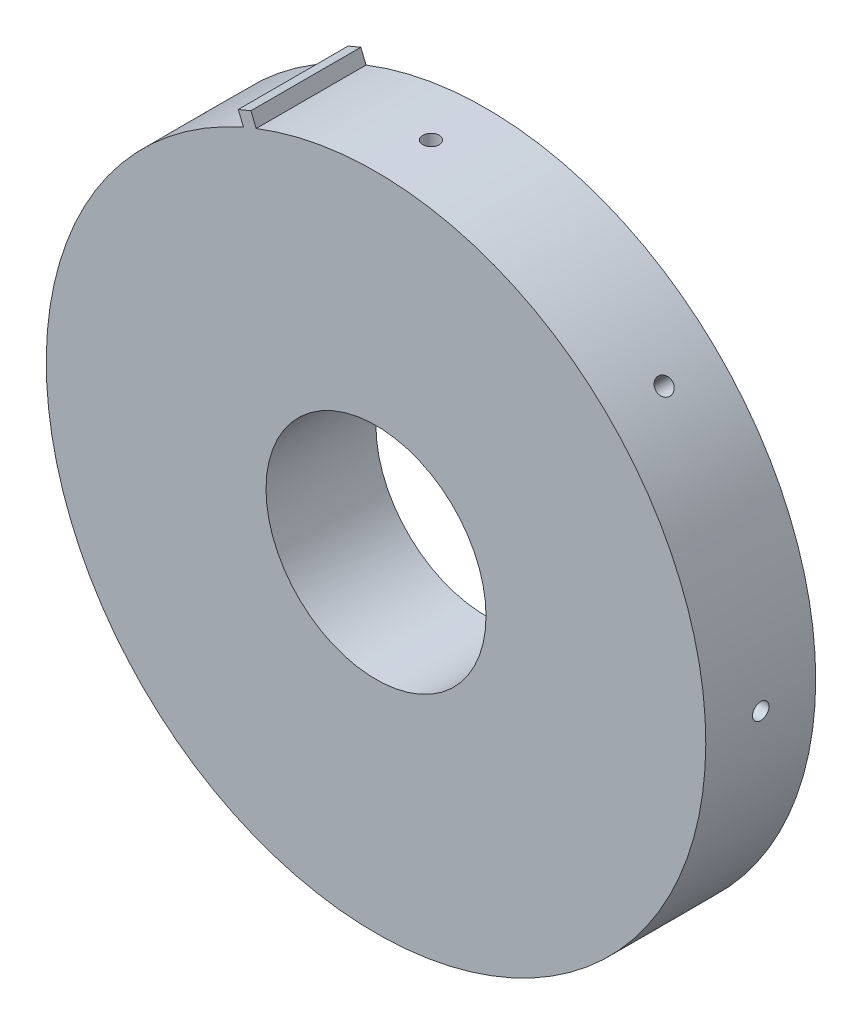
SolidWorks part; units mm, degrees
ref_plane "Front Plane" through (0, 0, 0) normal (0, 0, 1) x (1, 0, 0)
ref_plane "Top Plane" through (0, 0, 0) normal (0, 1, 0) x (1, 0, 0)
ref_plane "Right Plane" through (0, 0, 0) normal (1, 0, 0) x (0, 0, -1)
sketch "Sketch1" plane through (0, 0, 0) normal (0, 0, 1) x (1, 0, 0)
  circle A0 centre (0, 0) radius 40.03
  circle A1 centre (0, 0) radius 120
  dimension "D1" = 80.06
  dimension "D2" = 240
extrude "Boss-Extrude1" add sketch "Sketch1" along normal blind 40
sketch "Sketch2" plane through (0, 0, 0) normal (0, 0, -1) x (-1, 0, 0)
  circle A0 centre (0, 69.3) radius 2.655
  dimension "D2" = 5.31
extrude "Cut-Extrude1" cut sketch "Sketch2" against normal blind 10
sketch "Sketch3" plane through (0, 0, 10) normal (0, 0, -1) x (-1, 0, 0)
  circle A0 centre (0, 69.3) radius 3
  dimension "D1" = 6
extrude "Cut-Extrude3" cut sketch "Sketch3" against normal blind 10
sketch "Sketch5" plane through (0, 0, 20) normal (0, 0, -1) x (-1, 0, 0)
  line L0 (0, 72.3) -> (0, 66.3)
  arc A0 (0, 72.3) -> (0, 66.3) centre (0, 69.3) cw
  circle A1 centre (0, 69.3) radius 3 construction
revolve "Cut-Revolve1" cut sketch "Sketch5" angle 360 about L0
ref_plane "Plane2" through (0, 120, 0) normal (0, 1, 0) x (1, 0, 0)
sketch "Sketch6" plane through (0, 120, 0) normal (0, 1, 0) x (1, 0, 0)
  line L0 (-3, -20) -> (3, -20) construction
  circle A0 centre (0, -20) radius 3
extrude "Cut-Extrude4" cut sketch "Sketch6" against normal blind 50.7
pattern_circular "CirPattern1" count 8 over 360 about axis through (0, 0, 0) along (0, 0, 1) of "Cut-Extrude4", "Cut-Revolve1", "Cut-Extrude3", "Cut-Extrude1"
sketch "Sketch7" plane through (0, 0, 0) normal (0, 0, -1) x (-1, 0, 0)
  line L0 (0, 0) -> (0, 120)
  line L3 (45.5257, 116.4417) -> (50.1451, 114.5282)
  line L5 (50.1451, 114.5282) -> (47.7461, 108.7366)
  line L6 (43.1267, 110.65) -> (47.7461, 108.7366)
  line L7 (45.5257, 116.4417) -> (43.1267, 110.65)
  circle A0 centre (0, 0) radius 120 construction
extrude "Boss-Extrude2" add sketch "Sketch7" against normal blind 40 contours L3 L5 L6 L7
